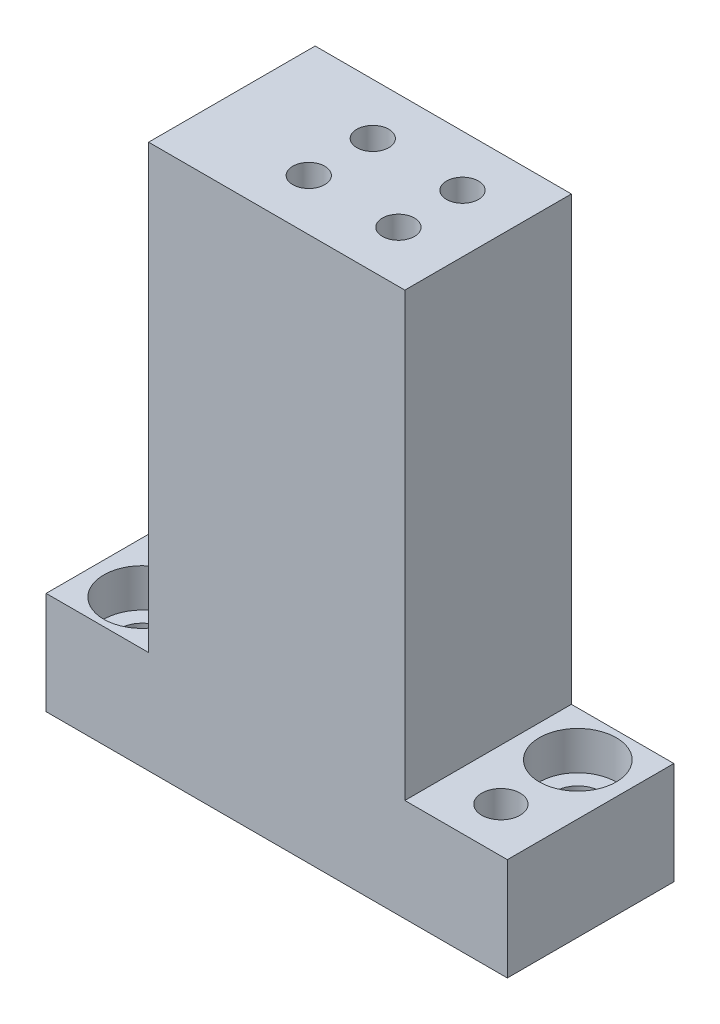
SolidWorks part; units mm, degrees
material "S45C"
ref_plane "Front" through (0, 0, 0) normal (0, 0, 1) x (1, 0, 0)
ref_plane "Top" through (0, 0, 0) normal (0, 1, 0) x (1, 0, 0)
ref_plane "Right" through (0, 0, 0) normal (1, 0, 0) x (0, 0, -1)
sketch "Sketch1" plane through (0, 0, 0) normal (0, 1, 0) x (1, 0, 0)
  line L1 (-36, 13) -> (36, 13)
  line L2 (-36, 13) -> (-36, -13)
  line L3 (-36, -13) -> (36, -13)
  line L4 (36, 13) -> (36, -13)
  line L5 (-36, 13) -> (36, -13) construction
  line L6 (-36, -13) -> (36, 13) construction
  point P0 (0, 0)
  dimension "D1" = 26
  dimension "D2" = 72
extrude "Boss-Extrude1" add sketch "Sketch1" along normal blind 16
sketch "Sketch2" plane through (0, 16, 0) normal (0, 1, 0) x (1, 0, 0)
  line L0 (-36, -13) -> (36, -13) construction
  line L1 (-20, 13) -> (20, 13)
  line L2 (-20, 13) -> (-20, -13)
  line L3 (-20, -13) -> (20, -13)
  line L4 (20, 13) -> (20, -13)
  line L5 (-20, 13) -> (20, -13) construction
  line L6 (-20, -13) -> (20, 13) construction
  point P0 (0, 0)
  dimension "D1" = 40
extrude "Boss-Extrude2" add sketch "Sketch2" along normal blind 69
sketch "Sketch3" plane through (0, 16, 0) normal (0, 1, 0) x (1, 0, 0)
  line L0 (36, 13) -> (20, 13) construction
  line L1 (36, -13) -> (36, 13) construction
  line L2 (-36, -13) -> (-20, -13) construction
  line L3 (-36, 13) -> (-36, -13) construction
  circle A0 centre (28, 6) radius 3.5
  circle A1 centre (28, -6) radius 3
  circle A2 centre (-28, -6) radius 3.5
  circle A3 centre (-28, 6) radius 3
  dimension "D7" = 7
  dimension "D8" = 6
  dimension "D1" = 12
  dimension "D2" = 12
  dimension "D3" = 7
  dimension "D4" = 8
  dimension "D5" = 7
  dimension "D6" = 8
extrude "Cut-Extrude1" cut sketch "Sketch3" against normal blind 96.5
sketch "Sketch4" plane through (0, 16, 0) normal (0, 1, 0) x (1, 0, 0)
  circle A0 centre (28, 6) radius 6
  circle A1 centre (-28, -6) radius 6
  dimension "D1" = 12
extrude "Cut-Extrude2" cut sketch "Sketch4" against normal blind 6
sketch "Sketch5" plane through (0, 85, 0) normal (0, 1, 0) x (1, 0, 0)
  line L0 (20, -13) -> (20, 13) construction
  line L1 (-3, 5) -> (11, 5) construction
  line L2 (-3, 5) -> (-3, -5) construction
  line L3 (-3, -5) -> (11, -5) construction
  line L4 (11, 5) -> (11, -5) construction
  line L5 (-3, 5) -> (11, -5) construction
  line L6 (-3, -5) -> (11, 5) construction
  circle A0 centre (-3, 5) radius 2.5
  circle A1 centre (11, 5) radius 2.5
  circle A2 centre (11, -5) radius 2.5
  circle A3 centre (-3, -5) radius 2.5
  point P0 (4, 0)
  dimension "D4" = 5
  dimension "D1" = 10
  dimension "D2" = 14
  dimension "D3" = 9
extrude "Cut-Extrude3" cut sketch "Sketch5" against normal blind 15
